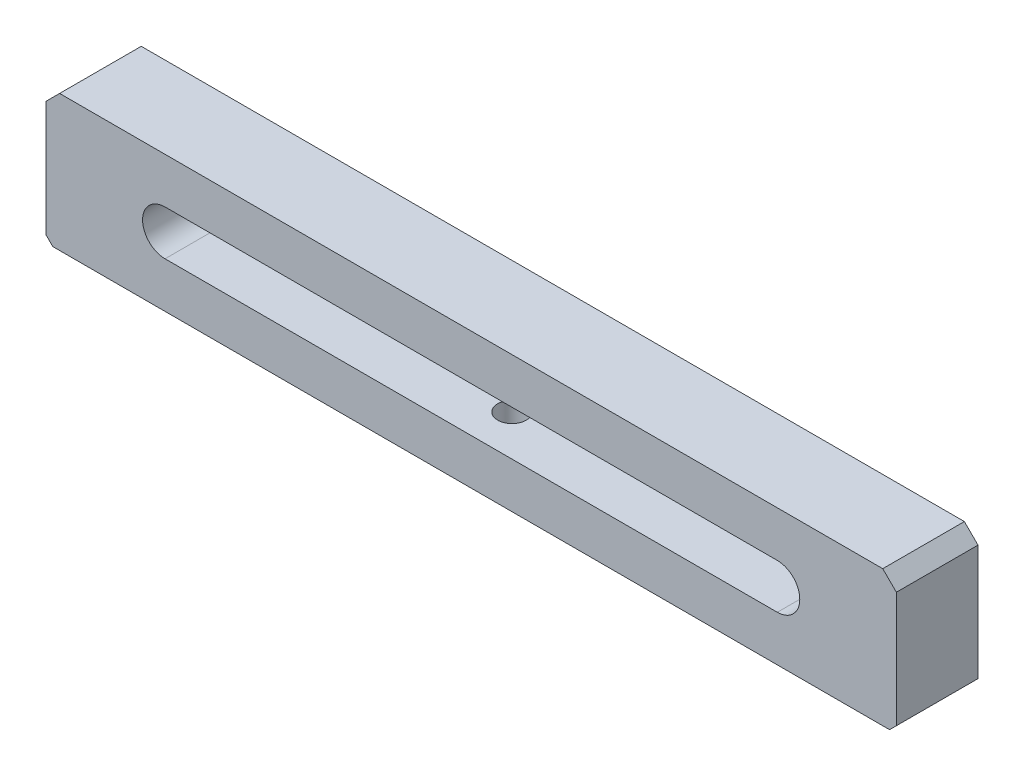
SolidWorks part; units mm, degrees
ref_plane "前视基准面" through (0, 0, 0) normal (0, 0, 1) x (1, 0, 0)
ref_plane "上视基准面" through (0, 0, 0) normal (0, 1, 0) x (1, 0, 0)
ref_plane "右视基准面" through (0, 0, 0) normal (1, 0, 0) x (0, 0, -1)
sketch "草图1" plane through (0, 0, 0) normal (0, 0, 1) x (1, 0, 0)
  line L1 (-62.5, -10) -> (62.5, -10)
  line L2 (-62.5, -10) -> (-62.5, 10)
  line L3 (-62.5, 10) -> (62.5, 10)
  line L4 (62.5, -10) -> (62.5, 10)
  line L5 (-62.5, -10) -> (62.5, 10) construction
  line L6 (-62.5, 10) -> (62.5, -10) construction
  point P0 (0, 0)
  dimension "D1" = 20
  dimension "D2" = 125
extrude "凸台-拉伸1" add sketch "草图1" along normal blind 12
sketch "草图2" plane through (0, 0, 12) normal (0, 0, 1) x (1, 0, 0)
  line L0 (-45, 0) -> (45, 0) construction
  line L1 (-45, 3.3) -> (45, 3.3)
  line L2 (-45, -3.3) -> (45, -3.3)
  line L3 (-62.5, -10) -> (62.5, -10) construction
  line L6 (0, 10) -> (0, 0) construction
  line L7 (62.5, 10) -> (-62.5, 10) construction
  arc A0 (-45, 3.3) -> (-45, -3.3) centre (-45, 0) ccw
  arc A1 (45, -3.3) -> (45, 3.3) centre (45, 0) ccw
  point P2 (0, 0)
  dimension "D1" = 90
  dimension "D2" = 6.6
  dimension "D3" = 10
extrude "切除-拉伸1" cut sketch "草图2" against normal through all
hole_wizard "M5 螺纹孔1" positions "草图3" profile "草图4" tap size "M5" standard "GB"
sketch "草图3" plane through (0, -10, 0) normal (0, -1, 0) x (-1, 0, 0)
  line L0 (0, 0) -> (0, -6) construction
  line L1 (62.5, 0) -> (-62.5, 0) construction
  point P0 (55, -6)
  point P2 (0, -6)
  point P4 (-55, -6)
  dimension "D1" = 110
  dimension "D2" = 6
sketch "草图4" plane through (-55, -10, 6) normal (1, 0, 0) x (0, 0, -1)
  line L0 (0, 0) -> (0, 11.2618)
  line L1 (0, 11.2618) -> (2.1, 10)
  line L2 (2.1, 10) -> (2.1, 0)
  line L5 (2.1, 0) -> (0, 0)
  line L10 (0, 11.2618) -> (-2.1, 10) construction
  line L11 (0, -6.35) -> (0, 107.95) construction
  dimension "螺纹孔钻头直径" = 4.2
  dimension "螺纹孔钻头深度" = 10
  dimension "导头角度" = 118
cosmetic thread "孔螺蚊线1" parameters "D1"=9.91, "D2"=5
cosmetic thread "孔螺蚊线2" parameters "D1"=6.7, "D2"=5
cosmetic thread "孔螺蚊线3" parameters "D1"=9.91, "D2"=5
chamfer "倒角1" distance 2 angle 45 2 edges at (-62.5, 10, 6) (62.5, 10, 6)
chamfer "倒角2" distance 1 angle 45 2 edges at (-62.5, -10, 6) (62.5, -10, 6)
